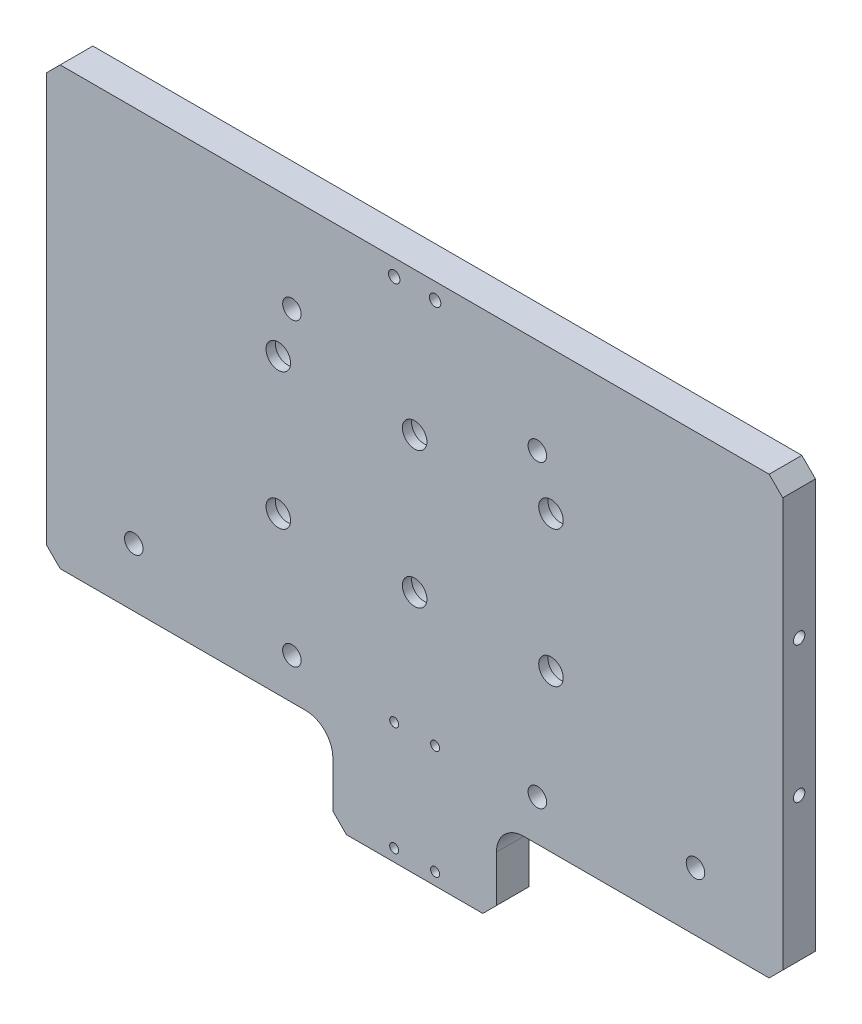
SolidWorks part; units mm, degrees
ref_plane "前视基准面" through (0, 0, 0) normal (0, 0, 1) x (1, 0, 0)
ref_plane "上视基准面" through (0, 0, 0) normal (0, 1, 0) x (1, 0, 0)
ref_plane "右视基准面" through (0, 0, 0) normal (1, 0, 0) x (0, 0, -1)
sketch "草图1" plane through (0, 0, 0) normal (0, 0, 1) x (1, 0, 0)
  line L1 (-135, 96) -> (135, 96)
  line L2 (-135, 96) -> (-135, -96)
  line L3 (-135, -96) -> (135, -96)
  line L4 (135, 96) -> (135, -96)
  line L5 (-135, 96) -> (135, -96) construction
  line L6 (-135, -96) -> (135, 96) construction
  point P0 (0, 0)
  dimension "D1" = 270
  dimension "D2" = 192
extrude "凸台-拉伸1" add sketch "草图1" along normal mid plane 12
sketch "草图2" plane through (0, 0, 6) normal (0, 0, 1) x (1, 0, 0)
  line L0 (0, 34.2365) -> (0, -132.3973) construction
  line L1 (-135, -96) -> (-30, -96)
  line L2 (-135, -96) -> (-135, -64)
  line L3 (-135, -64) -> (-30, -64)
  line L4 (-30, -96) -> (-30, -64)
  line L5 (135, -96) -> (135, -64)
  line L6 (30, -96) -> (30, -64)
  line L7 (135, -96) -> (30, -96)
  line L8 (135, -64) -> (30, -64)
  dimension "D1" = 105
  dimension "D2" = 32
extrude "切除-拉伸1" cut sketch "草图2" against normal blind 12
hole_wizard "M5 螺纹孔1" positions "草图4" profile "草图3" tap size "M5" standard "ISO"
sketch "草图4" plane through (0, 96, 0) normal (0, 1, 0) x (1, 0, 0)
  point P0 (-7.5, 0)
  point P2 (7.5, 0)
  dimension "D1" = 15
  dimension "D2" = 7.5
cosmetic thread "孔螺蚊线1" [suppressed] parameters "D1"=10, "D2"=5
cosmetic thread "孔螺蚊线2" [suppressed] parameters "D1"=10, "D2"=5
sketch "草图3" plane through (-7.5, 96, 0) normal (1, 0, 0) x (0, 0, 1)
  line L0 (0, 0) -> (0, 13.6618)
  line L1 (0, 13.6618) -> (2.1, 12.4)
  line L2 (2.1, 12.4) -> (2.1, 0)
  line L5 (2.1, 0) -> (0, 0)
  line L10 (0, 13.6618) -> (-2.1, 12.4) construction
  line L11 (0, -6.35) -> (0, 107.95) construction
  dimension "螺纹孔钻头直径" = 4.2
  dimension "螺纹孔钻头深度" = 12.4
  dimension "导头角度" = 118
hole_wizard "M8 螺纹孔1" positions "草图8" profile "草图7" tap size "M8" standard "ISO"
sketch "草图8" plane through (0, 0, 6) normal (0, 0, 1) x (1, 0, 0)
  line L1 (135, 96) -> (-135, 96) construction
  point P0 (-45, 61)
  point P16 (45, 61)
  dimension "D1" = 35
  dimension "D2" = 45
  dimension "D3" = 2
sketch "草图7" plane through (-45, 61, 6) normal (1, 0, 0) x (0, -1, 0)
  line L0 (0, 0) -> (0, 21.7929)
  line L1 (0, 21.7929) -> (3.4, 19.75)
  line L2 (3.4, 19.75) -> (3.4, 0)
  line L5 (3.4, 0) -> (0, 0)
  line L10 (0, 21.7929) -> (-3.4, 19.75) construction
  line L11 (0, -6.35) -> (0, 107.95) construction
  dimension "螺纹孔钻头直径" = 6.8
  dimension "螺纹孔钻头深度" = 19.75
  dimension "导头角度" = 118
cosmetic thread "孔螺蚊线3" parameters "D1"=12, "D2"=8
cosmetic thread "孔螺蚊线4" parameters "D1"=12, "D2"=8
hole_wizard "M4 螺纹孔1" positions "草图12" profile "草图11" tap size "M4" standard "ISO" end condition through all
sketch "草图12" plane through (0, 0, 6) normal (0, 0, 1) x (1, 0, 0)
  line L0 (-30, -96) -> (30, -96) construction
  point P0 (-7.5, -91.5)
  point P2 (7.5, -91.5)
  point P8 (-7.5, -51.5)
  point P10 (7.5, -51.5)
  dimension "D1" = 4.5
  dimension "D2" = 40
  dimension "D3" = 15
  dimension "D4" = 7.5
cosmetic thread "孔螺蚊线9" parameters "D2"=4
cosmetic thread "孔螺蚊线10" parameters "D2"=4
cosmetic thread "孔螺蚊线11" parameters "D2"=4
cosmetic thread "孔螺蚊线12" parameters "D2"=4
sketch "草图11" plane through (-7.5, -91.5, 6) normal (1, 0, 0) x (0, -1, 0)
  line L0 (0, 0) -> (0, 12)
  line L1 (0, 12) -> (1.65, 12)
  line L2 (1.65, 12) -> (1.65, 0)
  line L5 (1.65, 0) -> (0, 0)
  line L11 (0, -6.35) -> (0, 107.95) construction
  dimension "通孔螺纹孔钻头直径" = 3.3
  dimension "通孔螺纹孔钻头深度" = 12
chamfer "倒角1" distance 5 angle 45 6 edges at (-135, 96, 0) (135, 96, 0) (135, -64, 0) (30, -96, 0) (-30, -96, 0) (-135, -64, 0)
fillet "圆角1" radius 10 2 edges at (-30, -64, 0) (30, -64, 0)
hole_wizard "M8 六角凹头螺钉的柱形沉头孔2" positions "草图16" profile "草图15" counterbore size "M8" standard "ISO"
sketch "草图16" plane through (0, 0, -6) normal (0, 0, -1) x (-1, 0, 0)
  line L0 (0, 0) -> (0, 108.5781) construction
  line L2 (-130, 96) -> (130, 96) construction
  point P0 (31, 59.5)
  point P2 (-31, 59.5)
  point P4 (-31, 17.5)
  point P6 (31, 17.5)
  dimension "D1" = 62
  dimension "D2" = 36.5
  dimension "D3" = 42
sketch "草图15" plane through (-31, 59.5, -6) normal (1, 0, 0) x (0, 1, 0)
  line L0 (0, 0) -> (0, 12)
  line L1 (0, 12) -> (4.5, 12)
  line L3 (4.5, 12) -> (4.5, 8.6)
  line L4 (4.5, 8.6) -> (7.5, 8.6)
  line L5 (7.5, 8.6) -> (7.5, 0)
  line L7 (7.5, 0) -> (0, 0)
  line L11 (0, -6.35) -> (0, 107.95) construction
  dimension "通孔孔直径" = 9
  dimension "通孔孔深度" = 12
  dimension "柱形沉头孔直径" = 15
  dimension "柱形沉头孔深度" = 8.6
hole_wizard "M8 螺纹孔2" positions "草图18" profile "草图17" tap size "M8" standard "ISO" end condition through all
sketch "草图18" plane through (0, 0, -6) normal (0, 0, -1) x (-1, 0, 0)
  line L0 (0, 0) -> (0, -105.1634) construction
  line L2 (-130, -64) -> (-40, -64) construction
  line L3 (-130, 96) -> (130, 96) construction
  point P0 (-45, -49)
  point P2 (45, -49)
  point P4 (-103, -42.5)
  point P6 (103, -42.5)
  dimension "D1" = 90
  dimension "D2" = 206
  dimension "D3" = 21.5
  dimension "D4" = 145
sketch "草图17" plane through (45, -49, -6) normal (1, 0, 0) x (0, 1, 0)
  line L0 (0, 0) -> (0, 12)
  line L1 (0, 12) -> (3.4, 12)
  line L2 (3.4, 12) -> (3.4, 0)
  line L5 (3.4, 0) -> (0, 0)
  line L11 (0, -6.35) -> (0, 107.95) construction
  dimension "通孔螺纹孔钻头直径" = 6.8
  dimension "通孔螺纹孔钻头深度" = 12
cosmetic thread "孔螺蚊线13" parameters "D2"=8
cosmetic thread "孔螺蚊线14" parameters "D2"=8
cosmetic thread "孔螺蚊线15" parameters "D2"=8
cosmetic thread "孔螺蚊线16" parameters "D2"=8
hole_wizard "M8 六角凹头螺钉的柱形沉头孔3" positions "草图20" profile "草图19" counterbore size "M8" standard "ISO"
sketch "草图20" plane through (0, 0, -6) normal (0, 0, -1) x (-1, 0, 0)
  point P0 (-50, 43.5)
  point P3 (-50, -6.5)
  point P6 (0, 43.5)
  point P9 (0, -6.5)
  point P12 (50, 43.5)
  point P15 (50, -6.5)
sketch "草图19" plane through (50, 43.5, -6) normal (1, 0, 0) x (0, 1, 0)
  line L0 (0, 0) -> (0, 27.2039)
  line L1 (0, 27.2039) -> (4.5, 24.5)
  line L2 (4.5, 24.5) -> (4.5, 8.6)
  line L3 (4.5, 8.6) -> (7.5, 8.6)
  line L4 (7.5, 8.6) -> (7.5, 0)
  line L5 (7.5, 0) -> (0, 0)
  line L10 (0, 27.2039) -> (-4.5, 24.5) construction
  line L11 (0, -6.35) -> (0, 107.95) construction
  dimension "孔直径" = 9
  dimension "孔深度" = 24.5
  dimension "柱形沉头孔直径" = 15
  dimension "柱形沉头孔深度" = 8.6
  dimension "导头角度" = 118
hole_wizard "M5 螺纹孔2" positions "草图22" profile "草图21" tap size "M5" standard "ISO" end condition through all
sketch "草图22" plane through (0, 0, -6) normal (0, 0, -1) x (-1, 0, 0)
  line L0 (0, 0) -> (0, 107.8489) construction
  line L2 (-130, 96) -> (130, 96) construction
  point P0 (-7.5, 90)
  point P3 (7.5, 90)
  dimension "D1" = 15
  dimension "D2" = 6
sketch "草图21" plane through (7.5, 90, -6) normal (1, 0, 0) x (0, 1, 0)
  line L0 (0, 0) -> (0, 12)
  line L1 (0, 12) -> (2.1, 12)
  line L2 (2.1, 12) -> (2.1, 0)
  line L5 (2.1, 0) -> (0, 0)
  line L11 (0, -6.35) -> (0, 107.95) construction
  dimension "通孔螺纹孔钻头直径" = 4.2
  dimension "通孔螺纹孔钻头深度" = 12
cosmetic thread "孔螺蚊线17" parameters "D2"=5
cosmetic thread "孔螺蚊线18" parameters "D2"=5
hole_wizard "M5 螺纹孔3" positions "草图24" profile "草图23" tap size "M5" standard "ISO"
sketch "草图24" plane through (-135, 0, 0) normal (-1, 0, 0) x (0, 0, 1)
  line L0 (2, -6.5) -> (-2, -6.5) construction
  line L2 (-2, 43.5) -> (2, 43.5) construction
  point P0 (0, -6.5)
  point P2 (0, 43.5)
sketch "草图23" plane through (-135, -6.5, 0) normal (0, 1, 0) x (0, 0, 1)
  line L0 (0, 0) -> (0, 13.6618)
  line L1 (0, 13.6618) -> (2.1, 12.4)
  line L2 (2.1, 12.4) -> (2.1, 0)
  line L5 (2.1, 0) -> (0, 0)
  line L10 (0, 13.6618) -> (-2.1, 12.4) construction
  line L11 (0, -6.35) -> (0, 107.95) construction
  dimension "螺纹孔钻头直径" = 4.2
  dimension "螺纹孔钻头深度" = 12.4
  dimension "导头角度" = 118
cosmetic thread "孔螺蚊线19" parameters "D1"=10, "D2"=5
cosmetic thread "孔螺蚊线20" parameters "D1"=10, "D2"=5
ref_plane "基准面1" through (0, 0, 0) normal (1, 0, 0) x (0, 0, -1)
mirror "镜向1" about plane through (0, 0, 0) normal (1, 0, 0) of "M5 螺纹孔3"
